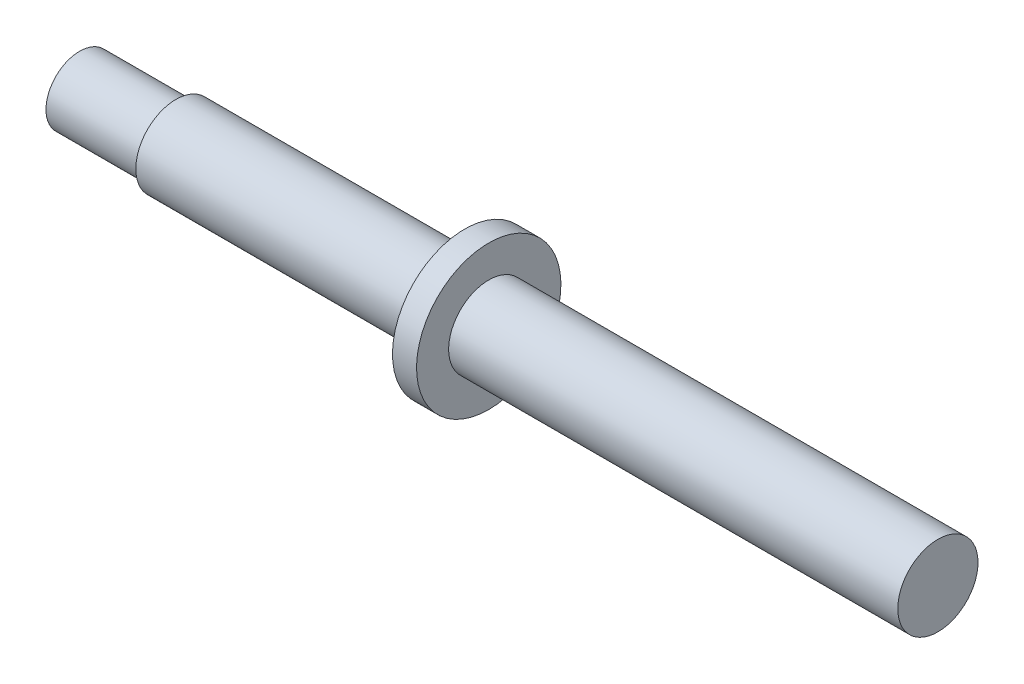
SolidWorks part; units mm, degrees
ref_plane "Front Plane" through (0, 0, 0) normal (0, 0, 1) x (1, 0, 0)
ref_plane "Top Plane" through (0, 0, 0) normal (0, 1, 0) x (1, 0, 0)
ref_plane "Right Plane" through (0, 0, 0) normal (1, 0, 0) x (0, 0, -1)
sketch "Sketch 1" plane through (0, 0, 0) normal (0, 0, 1) x (1, 0, 0)
  line L0 (0, 149.0741) -> (0, -207.4074) construction
  line L1 (-283.3333, 0) -> (255.5556, 0) construction
  line L2 (-187.5, 0) -> (-187.5, 25)
  line L3 (-187.5, 25) -> (-7.5, 25)
  line L4 (-7.5, 25) -> (-7.5, 45)
  line L5 (-7.5, 45) -> (7.5, 45)
  line L6 (-187.5, 0) -> (187.5, 0)
  line L7 (7.5, 25) -> (7.5, 45)
  line L8 (187.5, 25) -> (7.5, 25)
  line L9 (187.5, 0) -> (187.5, 25)
  point P12 (0, 0)
  point P13 (0, 45)
  dimension "D1" = 50
  dimension "D2" = 15
  dimension "D3" = 180
  dimension "D4" = 20
revolve "Revolve 1" add sketch "Sketch 1" angle 360 about L6
sketch "Sketch 2" plane through (187.5, 0, 0) normal (1, 0, 0) x (0, 0, -1)
  circle A1 centre (0, 0) radius 25
  circle A2 centre (0, 0) radius 25
  dimension "D1" = 0
extrude "Boss-Extrude 1" add sketch "Sketch 2" along normal blind 100
sketch "Sketch 3" plane through (-187.5, 0, 0) normal (-1, 0, 0) x (0, 0, 1)
  circle A0 centre (0, 0) radius 21
  dimension "D1" = 42
extrude "Boss-Extrude 2" add sketch "Sketch 3" along normal blind 60
